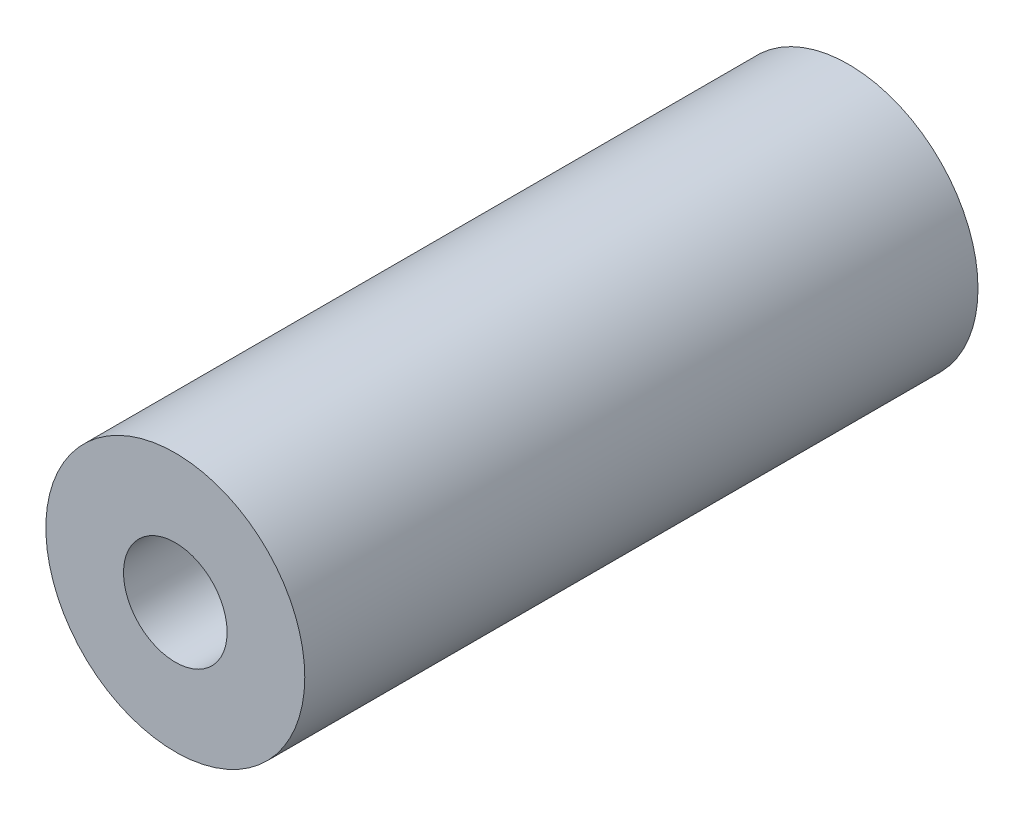
from build123d import *

# Parameters (mm, degrees)
SKETCH_1_R      = 5
SKETCH_1_R_2    = 2
EXTRUDE_1_DEPTH = 13


with BuildPart() as part:
    # 草图1 → 凸台-拉伸1 (new, symmetric)
    with BuildSketch(Plane.XY):
        Circle(SKETCH_1_R)
        Circle(SKETCH_1_R_2, mode=Mode.SUBTRACT)
    extrude(amount=EXTRUDE_1_DEPTH, both=True)


solid = part.part
